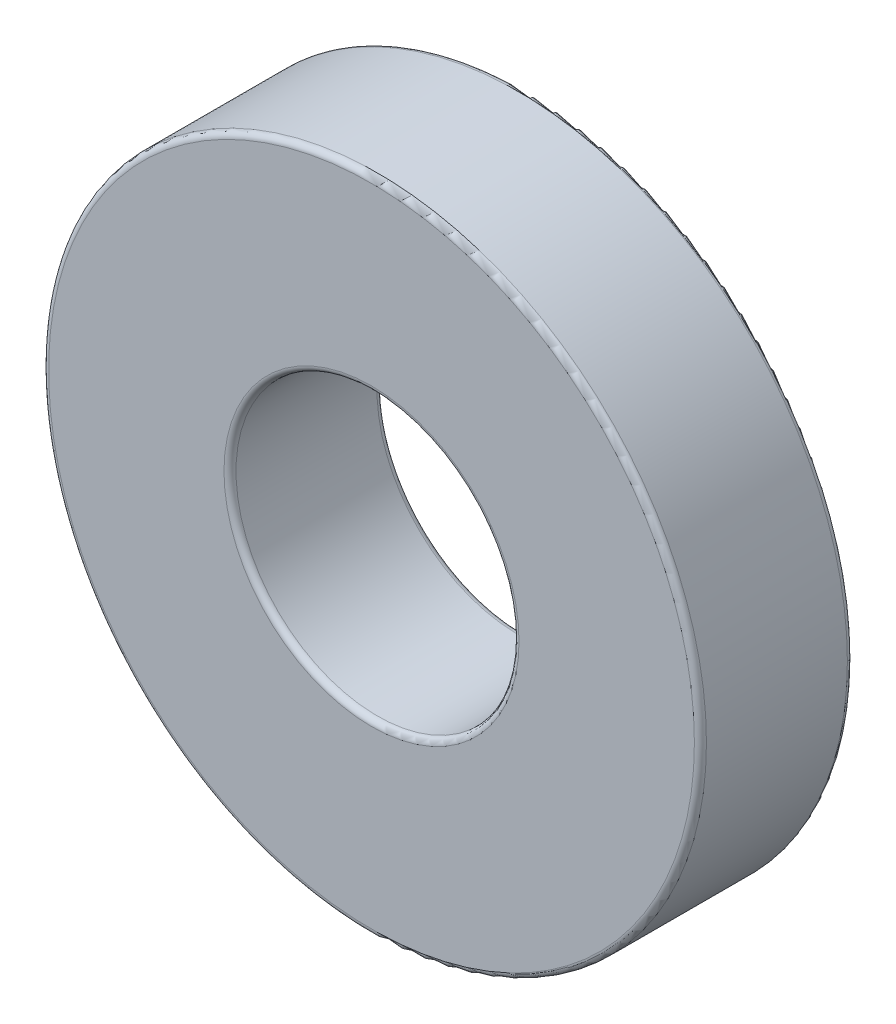
SolidWorks part; units mm, degrees
ref_plane "Front Plane" through (0, 0, 0) normal (0, 0, 1) x (1, 0, 0)
ref_plane "Top Plane" through (0, 0, 0) normal (0, 1, 0) x (1, 0, 0)
ref_plane "Right Plane" through (0, 0, 0) normal (1, 0, 0) x (0, 0, -1)
sketch "Sketch1" plane through (0, 0, 0) normal (0, 0, 1) x (1, 0, 0)
  circle A0 centre (0, 0) radius 117.475
  circle A1 centre (0, 0) radius 273.05
  dimension "D1" = 234.95
  dimension "D2" = 546.1
extrude "Boss-Extrude1" add sketch "Sketch1" along normal blind 127
fillet "Fillet1" radius 5 4 edges at (273.05, 0, 0) (117.475, 0, 0) (117.475, 0, 127) (273.05, 0, 127)
